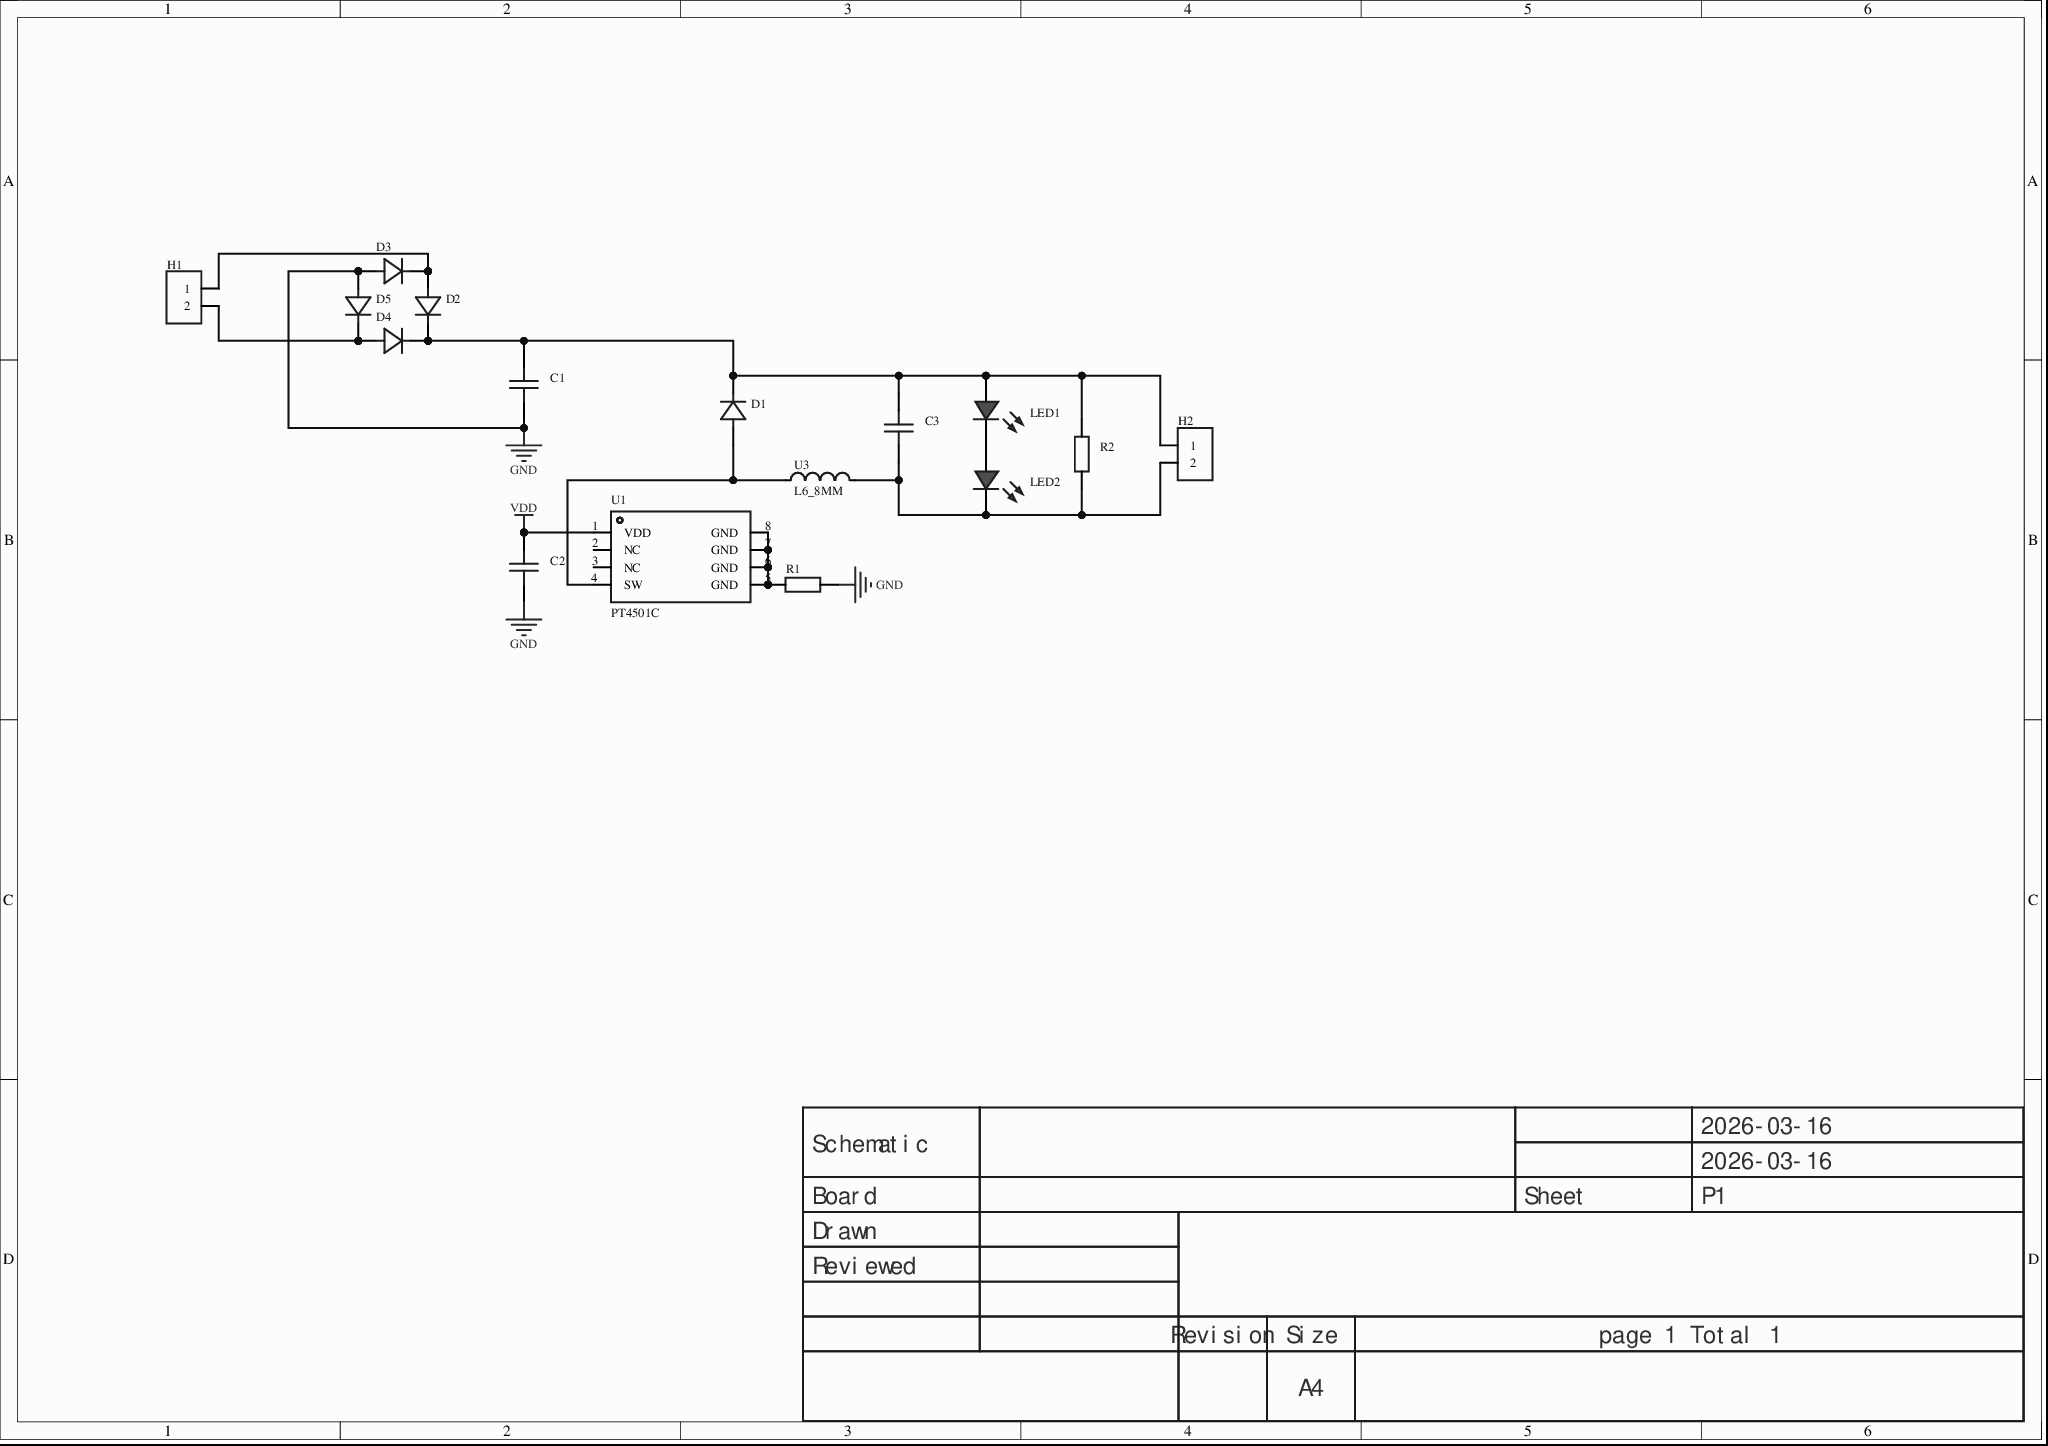
[diagram p0: MISC51823-3.schdoc]
# Altium project MISC51823-2.PrjPcb
1 sheet, 16 parts. Net scope: global (net labels, ports and power ports of the same name join across sheets).
Board file: MISC51823.pcbdoc

## Sheet MISC51823-3.schdoc
size 297 x 209 mm; Version: V1.0; @Project Name: MISC51823; @Update Date: 2026-03-16; @Create Date: 2026-03-16; @Board Name: MISC51823; @Create Time: 13:19:46; @Page Count: 1; @Page No: 1; @Schematic Name: MISC51823; @Update Time: 13:19:46; Size: A4

### Parts
C1  100nF  [CAP-TH_L5.0-W2.5-P5.00-D1.0]  (value not drawn)
C2  100nF  [CAP-TH_L5.0-W2.5-P5.00-D1.0]  (value not drawn)
C3  100nF  [CAP-TH_L5.0-W2.5-P5.00-D1.0]  (value not drawn)
D1  (no value)  [DO_1N4007]
D2  (no value)  [DO_1N4007]
D3  (no value)  [DO_1N4007]
D4  (no value)  [DO_1N4007]
D5  (no value)  [DO_1N4007]
H1  (no value)  [HDR-TH_2P-P2.54-V-F]
H2  (no value)  [HDR-TH_2P-P2.54-V-F]
LED1  (no value)  [LED_TH-3mm]
LED2  (no value)  [LED_TH-3mm]
R1  10kΩ  [Res_1/2W]  (value not drawn)
R2  10kΩ  [Res_1/2W]  (value not drawn)
U1  PT4501C  [SOP-8_L4.9-W3.9-P1.27-LS6.0-BL-EP]
U3  L6_8MM  [IND-TH_BD6.00-P3.00-D0.6]

### Nets
GND: C1.2 C2.2 D3.2(A) D5.2(A) R1.2
VDD: C2.1 U1.1(VDD)
NetC1_1: C1.1 C3.1 D1.1(K) D2.1(K) D4.1(K) H2.1 LED1.1(C) R2.2
NetC3_2: C3.2 H2.2 LED2.2(A) R2.1 U3.2
NetD1_2: D1.2(A) U1.4(SW) U3.1
NetD2_2: D2.2(A) D3.1(K) H1.1
NetD4_2: D4.2(A) D5.1(K) H1.2
NetLED1_2: LED1.2(A) LED2.1(C)
NetR1_1: R1.1 U1.5(GND) U1.6(GND) U1.7(GND) U1.8(GND)

Not connected (* = marked no-connect by the designer): U1 2(NC)* 3(NC)*

### Notes on the sheet
- 2026-03-16
- Schematic
- Board
- Sheet
- P1
- Drawn
- Reviewed
- Revision
- Size
- A4
- page 1 Total 1

### Library data of the parts
C1 = 100nF: Symbol: 100NF_C9900015256; 3D Model: 08e3d7481fc7486bb1b263873f51e1e10819f05c4eef4c71ace90d822a990e87; 3D Model Transform: 224.652,98.425,0,0,0,0,-0.005,0,-137.795; AddInBom: yes; ModelName: CAP-TH_BD5.0-W2.5-P5.08; Device: 100nF; LCSC Part Name: 100nF; Supplier Part: C9900015256; Manufacturer Part: 100nF; Supplier Footprint: CAP-TH_L5.0-W2.5-P5.00-D1.0; JLCPCB Part Class: Extended Part; Supplier: LCSC; ConvertToPcb: yes; FootprintName: CAP-TH_L5.0-W2.5-P5.00-D1.0
C2 C3 = 100nF: Symbol: 100NF_C9900015256; AddInBom: yes; ModelId: 08e3d7481fc7486bb1b263873f51e1e10819f05c4eef4c71ace90d822a990e87; ModelName: CAP-TH_BD5.0-W2.5-P5.08; ModelTransform: 224.652,98.425,0,0,0,0,-0.005,0,-137.795; Device: 100nF; LCSC Part Name: 100nF; SupplierPart: C9900015256; ManufacturerPart: 100nF; Supplier Footprint: CAP-TH_L5.0-W2.5-P5.00-D1.0; JLCPCB Part Class: Extended Part; Supplier: LCSC; ConvertToPcb: yes; FootprintName: CAP-TH_L5.0-W2.5-P5.00-D1.0
D1-D5 = D_1N4007A: AddInBom: yes; ModelId: 6de1e9b71a0d4751b4e9df530304c1a30819f05c4eef4c71ace90d822a990e87; ModelName: DO-41_D2.4-L4.7-P8.70; ModelTransform: 373.9,94.4,232.29,0,0,0,0,0,-140; Symbol: D_1N4007; Device: D_1N4007A; Supplier Footprint: DO-41; ConvertToPcb: yes; FootprintName: DO_1N4007
H1 H2 = HDR-F_2.54_1x2P: Symbol: Header-Female-2.54_1x2; ConvertToPcb: yes; ModelId: a9450ef445564560a104363b9aacde4e0819f05c4eef4c71ace90d822a990e87; ModelName: HDR-TH_2P-P2.54-F-LI-1X2P; ModelTransform: 215.7476,98.425,0,0,0,0,0,0,-129.921; Device: HDR-F_2.54_1x2P; AddInBom: yes; SupplierPart: C49661; Supplier Footprint: 插件; FootprintName: HDR-TH_2P-P2.54-V-F
LED1 LED2 = LED_TH-R_3mm: ConvertToPcb: yes; ModelId: a497c992633541038a38947cdc58012f0819f05c4eef4c71ace90d822a990e87; ModelName: LED-TH-3mm_R; ModelTransform: 141.274,153.327,0,0,0,0,-5.984,0,-137.795; Symbol: LED_TH-R; Device: LED_TH-R_3mm; AddInBom: yes; FootprintName: LED_TH-3mm; Supplier Footprint: 插件
R1 R2 = Res_AXIAL-1/2W: Symbol: Resistor; AddInBom: yes; ModelId: ba6d6a4d684e4c9c99cd35ba00f099d90819f05c4eef4c71ace90d822a990e87; ModelName: RES-TH_BD3.3-L9.0-P13.00-D0.6; ModelTransform: 535.33,129.8,326.71,0,0,0,0,0,-200; Device: Res_AXIAL-1/2W; Supplier Footprint: 轴向引线; ConvertToPcb: yes; FootprintName: Res_1/2W; Value: 10kΩ
U1 = PT4501C: component PT4501C componentd Dual-channel single-stage linear LED driver IC; Manufacturer: PowTech(华润矽威); AddInBom: yes; ModelId: 94c97984fe8342edbe821bc2ce85d11e0819f05c4eef4c71ace90d822a990e87; ModelName: SOP-8_L4.9-W3.9-H1.7-LS6.0-P1.30; ModelTransform: 236.22,839.658,0,90,0,0,0.0005,-0.0005,0; Symbol: PT4501C; Device: PT4501C; Manufacturer Part: PT4501C; LCSC Part Name: PT4501C; Supplier Footprint: SOP-8-EP; JLCPCB Part Class: Extended Part; Datasheet: https://atta.szlcsc.com/upload/public/pdf/source/20170818/C126166_1503051230151895237.pdf; Supplier: LCSC; ConvertToPcb: yes; FootprintName: SOP-8_L4.9-W3.9-P1.27-LS6.0-BL-EP
U3 = L6_8MM: AddInBom: yes; ModelId: 52be9a472e2c4e878b139b6202dbeead0819f05c4eef4c71ace90d822a990e87; ModelTransform: 236.22,236.22,0,0,0,0,-0.005,0,-196.85; Symbol: L6_8MM; Device: L6_8MM; LCSC Part Name: L6_8MM; SupplierPart: C9900023592; ManufacturerPart: L6_8MM; Supplier Footprint: 10uH0.5mm; JLCPCB Part Class: Extended Part; Supplier: LCSC; ConvertToPcb: yes; FootprintName: IND-TH_BD6.00-P3.00-D0.6; ModelName: IND-TH_BD6.00-P3.00-D0.6